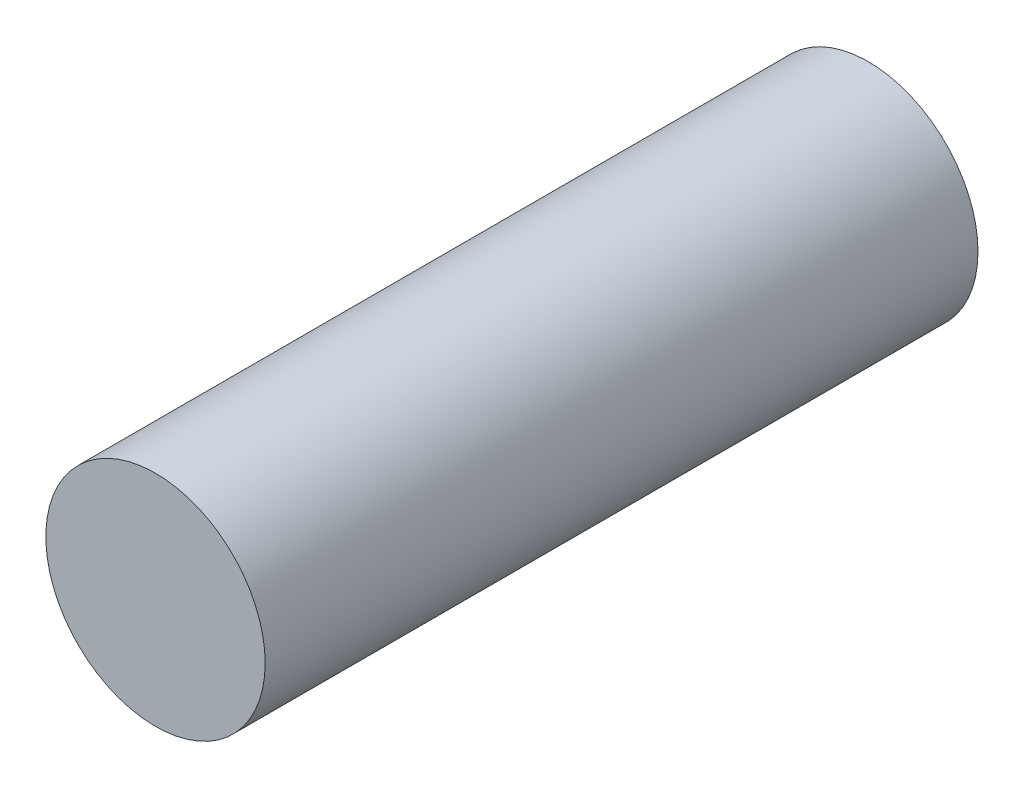
from build123d import *

# Parameters (mm, degrees)
SKETCH_1_R      = 10
EXTRUDE_1_DEPTH = 65


with BuildPart() as part:
    # 草图1 → 凸台-拉伸1 (new body)
    with BuildSketch(Plane.XY):
        Circle(SKETCH_1_R)
    extrude(amount=EXTRUDE_1_DEPTH)


solid = part.part
